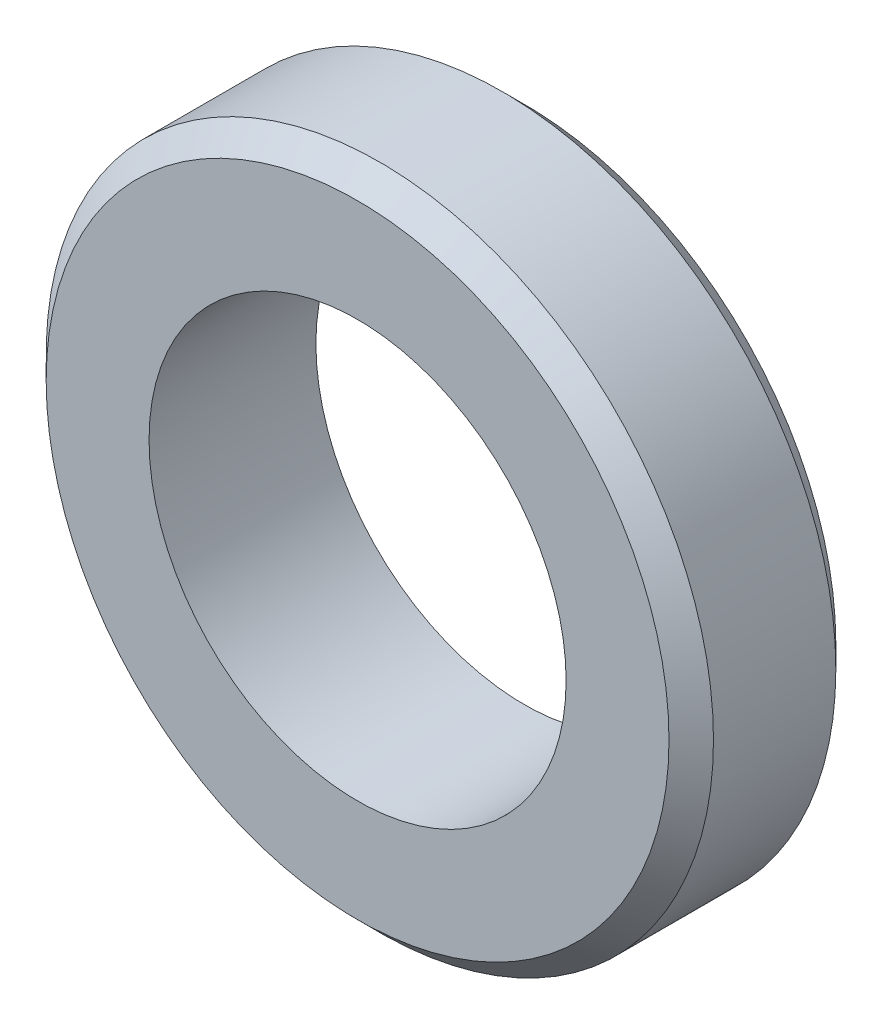
from build123d import *

# Parameters (mm, degrees)
SKETCH1_R              = 30
BOSS_EXTRUDE1_DEPTH    = 15
SKETCH2_R              = 17.5
CUT_EXTRUDE1_DEPTH     = 15
CHAMFER1_SIZE          = 2
M42_TAPPED_HOLE2_D     = 37.5
M42_TAPPED_HOLE2_DEPTH = 106.5
M42_TAPPED_HOLE2_TIP   = 11.266136607


with BuildPart() as part:
    # Sketch1 → Boss-Extrude1 (new body)
    with BuildSketch(Plane.XY):
        Circle(SKETCH1_R)
    extrude(amount=BOSS_EXTRUDE1_DEPTH)

    # Sketch2 → Cut-Extrude1 (cut)
    with BuildSketch(Plane.XY.offset(15)):
        Circle(SKETCH2_R)
    extrude(amount=-CUT_EXTRUDE1_DEPTH, mode=Mode.SUBTRACT)

    # Chamfer1
    chamfer1_edges = [part.edges().sort_by_distance(p)[0] for p in [
        (-30, 0, 0),
        (-30, 0, 15),
    ]]
    chamfer(chamfer1_edges, length=CHAMFER1_SIZE)

    # M42 Tapped Hole2
    with Locations(Plane.XY.offset(15)):
        with Locations((0, 0)):
            Hole(M42_TAPPED_HOLE2_D / 2, depth=M42_TAPPED_HOLE2_DEPTH)
            with Locations((0, 0, -(M42_TAPPED_HOLE2_DEPTH + M42_TAPPED_HOLE2_TIP / 2))):  # 118° drill point
                Cone(0, M42_TAPPED_HOLE2_D / 2, M42_TAPPED_HOLE2_TIP, mode=Mode.SUBTRACT)


solid = part.part
